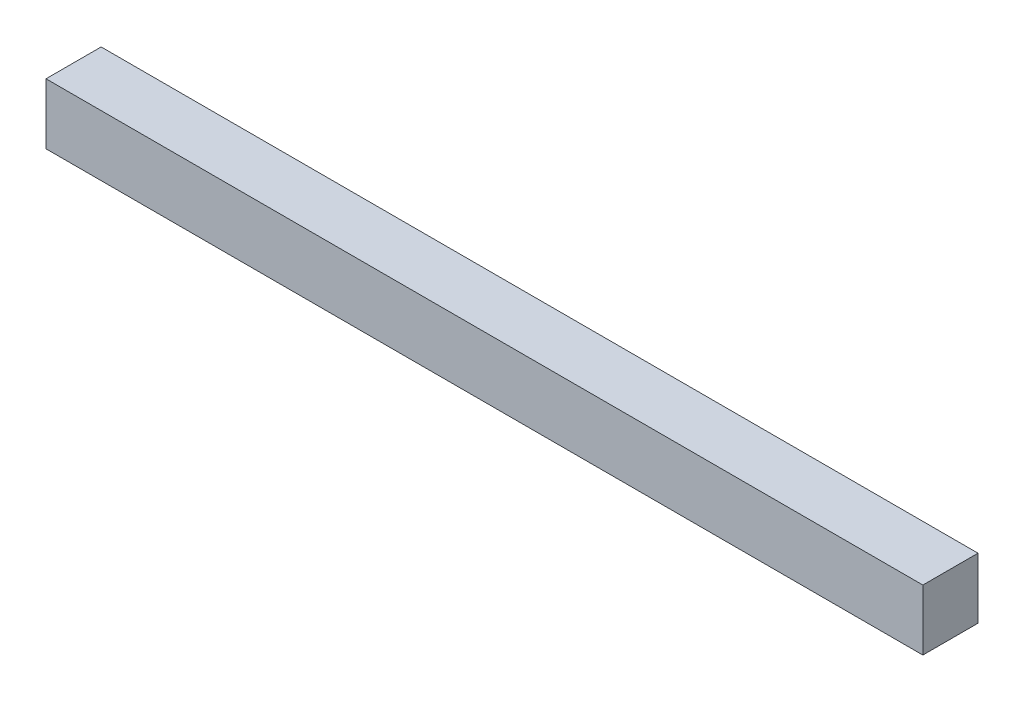
SolidWorks part; units mm, degrees
material "Q235B"
ref_plane "Front Plane" through (0, 0, 0) normal (0, 0, 1) x (1, 0, 0)
ref_plane "Top Plane" through (0, 0, 0) normal (0, 1, 0) x (1, 0, 0)
ref_plane "Right Plane" through (0, 0, 0) normal (1, 0, 0) x (0, 0, -1)
sketch "Sketch1" plane through (0, 0, 0) normal (0, 0, 1) x (1, 0, 0)
  line L1 (0, 0) -> (318, 0)
  line L2 (0, 0) -> (0, 22)
  line L3 (0, 22) -> (318, 22)
  line L4 (318, 0) -> (318, 22)
  dimension "D1" = 318
  dimension "D2" = 22
extrude "Boss-Extrude1" add sketch "Sketch1" along normal blind 20
